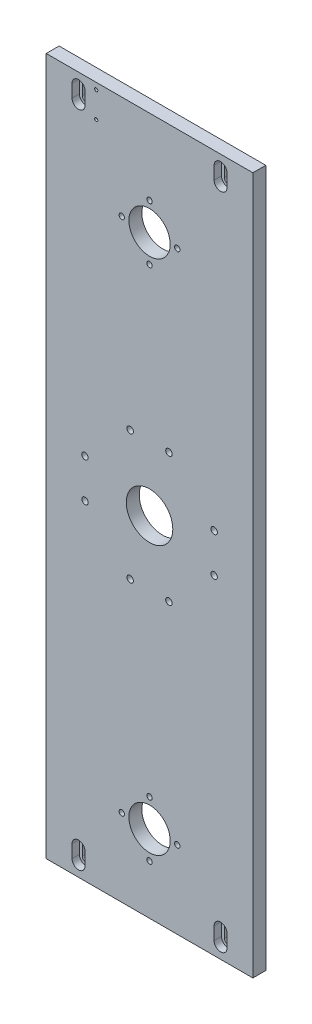
from build123d import *

# Parameters (mm, degrees)
SKETCH_1_W                = 160
SKETCH_1_H                = 540
EXTRUDE_1_DEPTH           = 10
SKETCH_2_R                = 16
CUT_EXTRUDE_1_DEPTH       = 282.780056072
SKETCH_3_R                = 18
CUT_EXTRUDE_2_DEPTH       = 282.780056072
HOLE_WIZARD_1_D           = 5.5
HOLE_WIZARD_1_CBORE_D     = 10
HOLE_WIZARD_1_CBORE_DEPTH = 5.7
HOLE_WIZARD_M5_1_D        = 4.2
HOLE_WIZARD_M5_2_D        = 4.2
HOLE_WIZARD_M5_3_D        = 4.2
HOLE_WIZARD_M3_1_D        = 2.5
HOLE_WIZARD_M6_2_D        = 5
CUT_EXTRUDE_3_DEPTH       = 5.7
CUT_EXTRUDE_4_DEPTH       = 282.660238585
HOLE_WIZARD_M6_3_D        = 5


with BuildPart() as part:
    # 草图1 → 凸台-拉伸1 (new body)
    with BuildSketch(Plane.XY):
        Rectangle(SKETCH_1_W, SKETCH_1_H)
    extrude(amount=EXTRUDE_1_DEPTH)

    # 草图2 → 切除-拉伸1 (cut, through all)
    with BuildSketch(Plane.XY.offset(10)):
        with Locations((0, 190)):
            Circle(SKETCH_2_R)
        with Locations((0, -210)):
            Circle(SKETCH_2_R)
    extrude(amount=-CUT_EXTRUDE_1_DEPTH, mode=Mode.SUBTRACT)

    # 草图3 → 切除-拉伸2 (cut, through all)
    with BuildSketch(Plane.XY.offset(10)):
        Circle(SKETCH_3_R)
    extrude(amount=-CUT_EXTRUDE_2_DEPTH, mode=Mode.SUBTRACT)

    # 打孔尺寸根据内六角圆柱头螺钉的类型1 (through all)
    with Locations(Plane.XY.offset(10)):
        with Locations((-55, 255), (55, 255), (55, -255), (-55, -255)):
            CounterBoreHole(HOLE_WIZARD_1_D / 2, HOLE_WIZARD_1_CBORE_D / 2, HOLE_WIZARD_1_CBORE_DEPTH)

    # M5 螺纹孔1 (through all)
    with Locations(Plane.XY.offset(10)):
        with Locations((0, 211.5)):
            Hole(HOLE_WIZARD_M5_1_D / 2)

    # M5 螺纹孔2 (through all)
    with Locations(Plane.XY.offset(10)):
        with Locations((0, -231.5)):
            Hole(HOLE_WIZARD_M5_2_D / 2)

    # M5 螺纹孔3 (through all)
    with Locations(Plane.XY.offset(10)):
        with Locations((21.5, -210), (-21.5, -210), (0, -188.5), (-21.5, 190), (21.5, 190), (0, 168.5)):
            Hole(HOLE_WIZARD_M5_3_D / 2)

    # M3 螺纹孔1 (through all)
    with Locations(Plane.XY.offset(10)):
        with Locations((-41.3, 265), (-41.3, 245)):
            Hole(HOLE_WIZARD_M3_1_D / 2)

    # M6 螺纹孔2 (through all)
    with Locations(Plane(origin=(0, 0, 0), x_dir=(-1, 0, 0), z_dir=(0, 0, -1))):
        with Locations((-50, 15), (-50, -15), (50, 15), (50, -15)):
            Hole(HOLE_WIZARD_M6_2_D / 2)

    # 草图24 → 切除-拉伸3 (cut)
    with BuildSketch(Plane.XY.offset(10)):
        with BuildLine():
            Line((-50, 260), (-50, 250))
            ThreePointArc((-50, 250), (-55, 245), (-60, 250))
            Line((-60, 250), (-60, 260))
            ThreePointArc((-60, 260), (-55, 265), (-50, 260))
        make_face()
        with BuildLine():
            Line((60, 260), (60, 250))
            ThreePointArc((60, 250), (55, 245), (50, 250))
            Line((50, 250), (50, 260))
            ThreePointArc((50, 260), (55, 265), (60, 260))
        make_face()
        with BuildLine():
            Line((-50, -250), (-50, -260))
            ThreePointArc((-50, -260), (-55, -265), (-60, -260))
            Line((-60, -260), (-60, -250))
            ThreePointArc((-60, -250), (-55, -245), (-50, -250))
        make_face()
        with BuildLine():
            Line((60, -250), (60, -260))
            ThreePointArc((60, -260), (55, -265), (50, -260))
            Line((50, -260), (50, -250))
            ThreePointArc((50, -250), (55, -245), (60, -250))
        make_face()
    extrude(amount=-CUT_EXTRUDE_3_DEPTH, mode=Mode.SUBTRACT)

    # 草图25 → 切除-拉伸4 (cut, through all)
    with BuildSketch(Plane.XY.offset(4.3)):
        with BuildLine():
            Line((-52.25, 260), (-52.25, 250))
            ThreePointArc((-52.25, 250), (-55, 247.25), (-57.75, 250))
            Line((-57.75, 250), (-57.75, 260))
            ThreePointArc((-57.75, 260), (-55, 262.75), (-52.25, 260))
        make_face()
        with BuildLine():
            Line((57.75, 260), (57.75, 250))
            ThreePointArc((57.75, 250), (55, 247.25), (52.25, 250))
            Line((52.25, 250), (52.25, 260))
            ThreePointArc((52.25, 260), (55, 262.75), (57.75, 260))
        make_face()
        with BuildLine():
            Line((-52.25, -250), (-52.25, -260))
            ThreePointArc((-52.25, -260), (-55, -262.75), (-57.75, -260))
            Line((-57.75, -260), (-57.75, -250))
            ThreePointArc((-57.75, -250), (-55, -247.25), (-52.25, -250))
        make_face()
        with BuildLine():
            Line((57.75, -250), (57.75, -260))
            ThreePointArc((57.75, -260), (55, -262.75), (52.25, -260))
            Line((52.25, -260), (52.25, -250))
            ThreePointArc((52.25, -250), (55, -247.25), (57.75, -250))
        make_face()
    extrude(amount=-CUT_EXTRUDE_4_DEPTH, mode=Mode.SUBTRACT)

    # M6 螺纹孔3 (through all)
    with Locations(Plane(origin=(0, 0, 0), x_dir=(-1, 0, 0), z_dir=(0, 0, -1))):
        with Locations((15, -50), (-15, -50), (-15, 50), (15, 50)):
            Hole(HOLE_WIZARD_M6_3_D / 2)


solid = part.part
